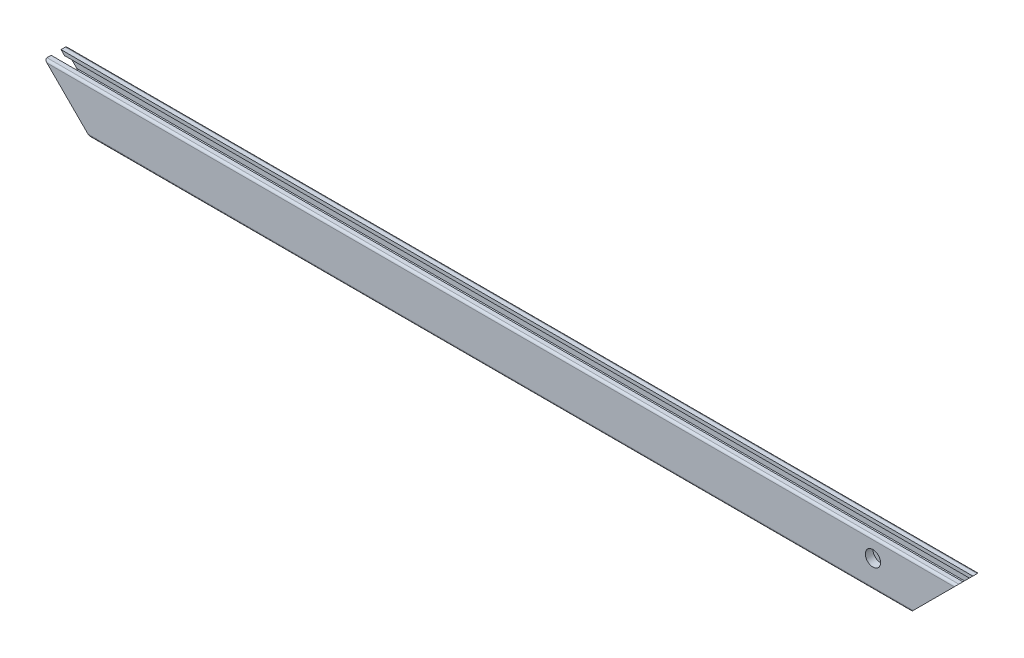
SolidWorks part; units mm, degrees
ref_plane "前视" through (0, 0, 0) normal (0, 0, 1) x (1, 0, 0)
ref_plane "上视" through (0, 0, 0) normal (0, 1, 0) x (1, 0, 0)
ref_plane "右视" through (0, 0, 0) normal (1, 0, 0) x (0, 0, -1)
sketch3d "3D草图1"
  line L0 (-300, 0, 0) -> (300, 0, 0)
  dimension "D1" = 600
other "结构构件1"
ref_plane "基准面1" through (-300, 0, 0) normal (1, 0, 0) x (0, 0, -1)
sketch "Sketch12" plane through (-300, 0, 0) normal (1, 0, 0) x (0, 0, -1)
  line L1 (0, 16.311) -> (0, -16.311) construction
  line L2 (0, 0) -> (9.513, 0) construction
  line L3 (-6, -15) -> (-3.25, -15)
  line L4 (-7.5, -13.5) -> (-7.5, 13.5)
  line L5 (-6, 15) -> (-3.25, 15)
  line L6 (7.5, -13.5) -> (7.5, 13.5)
  line L17 (3.25, 15) -> (6, 15)
  line L20 (-5.7, 12.7) -> (-5.7, 7)
  line L21 (-3.25, 12.7) -> (-5.7, 12.7)
  line L24 (5.7, 12.7) -> (5.7, 7)
  line L25 (3.25, 12.7) -> (5.7, 12.7)
  line L26 (-3.25, 15) -> (-3.25, 12.7)
  line L27 (3.25, 15) -> (3.25, 12.7)
  line L40 (5.7, -12.7) -> (5.7, -7)
  line L41 (3.25, -12.7) -> (5.7, -12.7)
  line L44 (-5.7, -12.7) -> (-5.7, -7)
  line L45 (-3.25, -12.7) -> (-5.7, -12.7)
  line L47 (3.25, -15) -> (3.25, -12.7)
  line L48 (-3.25, -15) -> (-3.25, -12.7)
  line L49 (3.25, -15) -> (6, -15)
  arc A0 (-6, -15) -> (-7.5, -13.5) centre (-6, -13.5) cw
  arc A1 (6, -15) -> (7.5, -13.5) centre (6, -13.5) ccw
  arc A2 (6, 15) -> (7.5, 13.5) centre (6, 13.5) cw
  arc A3 (-7.5, 13.5) -> (-6, 15) centre (-6, 13.5) cw
  circle A4 centre (0, 0) radius 2.5
  arc A5 (-5.7, 7) -> (5.7, 7) centre (0, 12.248) ccw
  arc A6 (-5.7, -7) -> (5.7, -7) centre (0, -12.248) cw
  point P4 (0, 0)
  point P21 (0, 0)
  point P44 (-7.5, 15)
  point P45 (7.5, 15)
  point P46 (7.5, -15)
  point P47 (-7.5, -15)
  point P48 (0, -15)
  point P49 (0, 15)
  dimension "D1" = 30
  dimension "D2" = 15
  dimension "D3" = 1.5
  dimension "D4" = 5
  dimension "D5" = 6.5
  dimension "D6" = 10.5
  dimension "D7" = 8
  dimension "D8" = 11.4
  dimension "D9" = 2.3
sketch "草图4" plane through (0, 0, 7.5) normal (0, 0, 1) x (1, 0, 0)
  line L0 (-300, 15) -> (-270, -15)
  line L2 (0, 0) -> (0, -85.0329) construction
  line L3 (-270, -15) -> (-300, -15)
  line L4 (-300, -15) -> (-300, 15)
  line L5 (300, -15) -> (300, 15)
  line L6 (270, -15) -> (300, -15)
  line L7 (300, 15) -> (270, -15)
  line L8 (300, 15) -> (-300, 15) construction
  line L9 (300, -15) -> (-300, -15) construction
  line L10 (-300, 13.5) -> (-300, -13.5) construction
extrude "切除-拉伸1" cut sketch "草图4" against normal through all
sketch "草图7" plane through (0, 0, 7.5) normal (0, 0, 1) x (1, 0, 0)
  line L0 (300, 15) -> (-300, 15) construction
  circle A0 centre (245, 3) radius 5
  dimension "D1" = 10
  dimension "D2" = 55
  dimension "D3" = 12
extrude "切除-拉伸2" cut sketch "草图7" against normal blind 4.999
